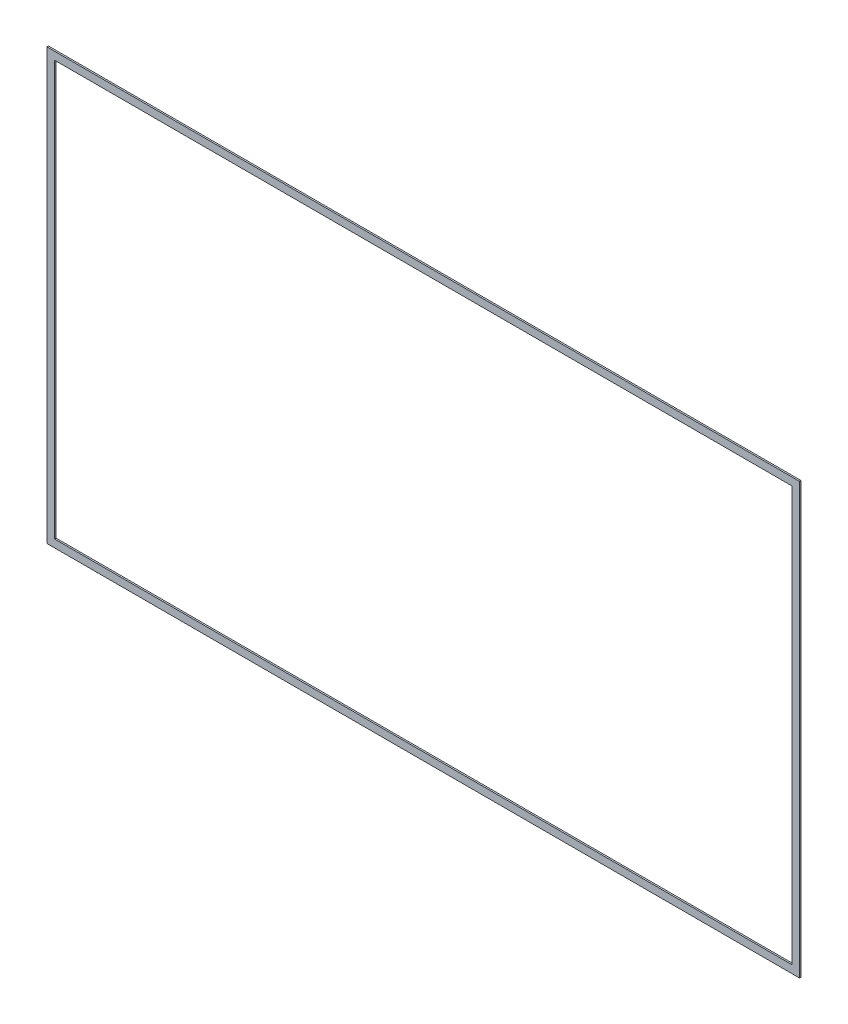
SolidWorks part; units mm, degrees
ref_plane "前视基准面" through (0, 0, 0) normal (0, 0, 1) x (1, 0, 0)
ref_plane "上视基准面" through (0, 0, 0) normal (0, 1, 0) x (1, 0, 0)
ref_plane "右视基准面" through (0, 0, 0) normal (1, 0, 0) x (0, 0, -1)
sketch "草图1" plane through (0, 0, 0) normal (0, 0, 1) x (1, 0, 0)
  line L0 (-487.3, -278.5) -> (487.3, -278.5)
  line L5 (-477.3, 268.5) -> (477.3, 268.5)
  line L6 (-477.3, 268.5) -> (-477.3, -268.5)
  line L7 (-477.3, -268.5) -> (477.3, -268.5)
  line L8 (477.3, 268.5) -> (477.3, -268.5)
  line L9 (-477.3, 268.5) -> (477.3, -268.5) construction
  line L10 (-477.3, -268.5) -> (477.3, 268.5) construction
  line L11 (487.3, 278.5) -> (487.3, -278.5)
  line L12 (-487.3, 278.5) -> (487.3, 278.5)
  line L13 (-487.3, 278.5) -> (-487.3, -278.5)
  point P0 (0, 0)
  dimension "D1" = 954.6
  dimension "D2" = 537
  dimension "D3" = 10
extrude "凸台-拉伸1" add sketch "草图1" along normal blind 2
fillet "圆角1" radius 0.2 4 edges at (-477.3, -268.5, 1) (-477.3, 268.5, 1) (477.3, 268.5, 1) (477.3, -268.5, 1)
